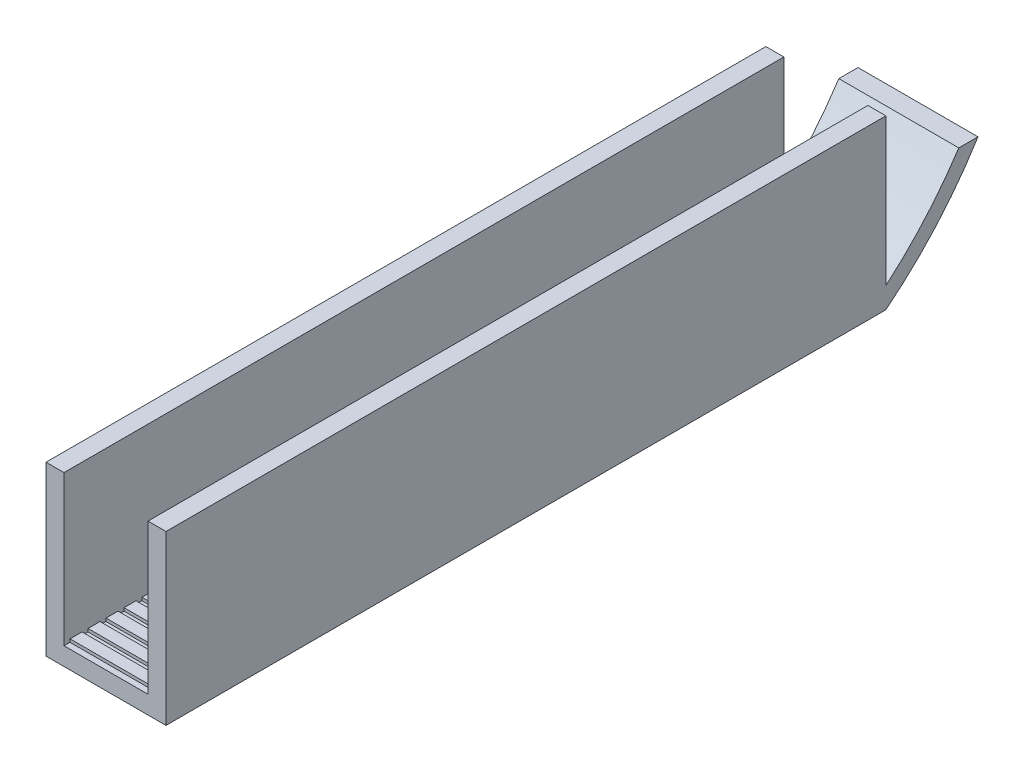
from build123d import *

# Parameters (mm, degrees)
SKETCH1_W           = 200
SKETCH1_H           = 30
BOSS_EXTRUDE1_DEPTH = 1200
SKETCH2_W           = 200
SKETCH2_H           = 20
BOSS_EXTRUDE2_DEPTH = 5
BOSS_EXTRUDE3_DEPTH = 200
SKETCH5_W           = 30
SKETCH5_H           = 1200
BOSS_EXTRUDE5_DEPTH = 250


with BuildPart() as part:
    # Sketch1 → Boss-Extrude1 (new body)
    with BuildSketch(Plane.XY):
        with Locations((-100, 15)):
            Rectangle(SKETCH1_W, SKETCH1_H)
    extrude(amount=BOSS_EXTRUDE1_DEPTH)

    # Sketch2 → Boss-Extrude2 (add)
    with BuildSketch(Plane(origin=(0, 30, 0), x_dir=(1, 0, 0), z_dir=(0, 1, 0))):
        with Locations((-100, -10)):
            Rectangle(SKETCH2_W, SKETCH2_H)
        with Locations((-100, -40)):
            Rectangle(SKETCH2_W, SKETCH2_H)
        with Locations((-100, -70)):
            Rectangle(SKETCH2_W, SKETCH2_H)
        with Locations((-100, -100)):
            Rectangle(SKETCH2_W, SKETCH2_H)
        with Locations((-100, -130)):
            Rectangle(SKETCH2_W, SKETCH2_H)
        with Locations((-100, -160)):
            Rectangle(SKETCH2_W, SKETCH2_H)
        with Locations((-100, -190)):
            Rectangle(SKETCH2_W, SKETCH2_H)
        with Locations((-100, -220)):
            Rectangle(SKETCH2_W, SKETCH2_H)
        with Locations((-100, -250)):
            Rectangle(SKETCH2_W, SKETCH2_H)
        with Locations((-100, -280)):
            Rectangle(SKETCH2_W, SKETCH2_H)
        with Locations((-100, -310)):
            Rectangle(SKETCH2_W, SKETCH2_H)
        with Locations((-100, -340)):
            Rectangle(SKETCH2_W, SKETCH2_H)
        with Locations((-100, -370)):
            Rectangle(SKETCH2_W, SKETCH2_H)
        with Locations((-100, -400)):
            Rectangle(SKETCH2_W, SKETCH2_H)
        with Locations((-100, -430)):
            Rectangle(SKETCH2_W, SKETCH2_H)
        with Locations((-100, -460)):
            Rectangle(SKETCH2_W, SKETCH2_H)
        with Locations((-100, -490)):
            Rectangle(SKETCH2_W, SKETCH2_H)
        with Locations((-100, -520)):
            Rectangle(SKETCH2_W, SKETCH2_H)
        with Locations((-100, -550)):
            Rectangle(SKETCH2_W, SKETCH2_H)
        with Locations((-100, -580)):
            Rectangle(SKETCH2_W, SKETCH2_H)
        with Locations((-100, -610)):
            Rectangle(SKETCH2_W, SKETCH2_H)
        with Locations((-100, -640)):
            Rectangle(SKETCH2_W, SKETCH2_H)
        with Locations((-100, -670)):
            Rectangle(SKETCH2_W, SKETCH2_H)
        with Locations((-100, -700)):
            Rectangle(SKETCH2_W, SKETCH2_H)
        with Locations((-100, -730)):
            Rectangle(SKETCH2_W, SKETCH2_H)
        with Locations((-100, -760)):
            Rectangle(SKETCH2_W, SKETCH2_H)
        with Locations((-100, -790)):
            Rectangle(SKETCH2_W, SKETCH2_H)
        with Locations((-100, -820)):
            Rectangle(SKETCH2_W, SKETCH2_H)
        with Locations((-100, -850)):
            Rectangle(SKETCH2_W, SKETCH2_H)
        with Locations((-100, -880)):
            Rectangle(SKETCH2_W, SKETCH2_H)
        with Locations((-100, -910)):
            Rectangle(SKETCH2_W, SKETCH2_H)
        with Locations((-100, -940)):
            Rectangle(SKETCH2_W, SKETCH2_H)
        with Locations((-100, -970)):
            Rectangle(SKETCH2_W, SKETCH2_H)
        with Locations((-100, -1000)):
            Rectangle(SKETCH2_W, SKETCH2_H)
        with Locations((-100, -1030)):
            Rectangle(SKETCH2_W, SKETCH2_H)
        with Locations((-100, -1060)):
            Rectangle(SKETCH2_W, SKETCH2_H)
        with Locations((-100, -1090)):
            Rectangle(SKETCH2_W, SKETCH2_H)
        with Locations((-100, -1120)):
            Rectangle(SKETCH2_W, SKETCH2_H)
        with Locations((-100, -1150)):
            Rectangle(SKETCH2_W, SKETCH2_H)
        with Locations((-100, -1180)):
            Rectangle(SKETCH2_W, SKETCH2_H)
    extrude(amount=BOSS_EXTRUDE2_DEPTH)

    # Sketch3 → Boss-Extrude3 (add)
    with BuildSketch(Plane(origin=(0, 0, 0), x_dir=(0, 0, -1), z_dir=(1, 0, 0))):
        with BuildLine():
            Line((121.535209025, 172.957157936), (153.547498251, 172.957157936))
            ThreePointArc((153.547498251, 172.957157936), (84.214276957, 79.873044696), (0, 0))
            Line((0, 0), (-44.824767416, 0))
            ThreePointArc((-44.824767416, 0), (46.406337039, 78.734560026), (121.535209025, 172.957157936))
        make_face()
    extrude(amount=-BOSS_EXTRUDE3_DEPTH)

    # Sketch5 → Boss-Extrude5 (add)
    with BuildSketch(Plane(origin=(0, 30, 0), x_dir=(1, 0, 0), z_dir=(0, 1, 0))):
        with Locations((-185, -600)):
            Rectangle(SKETCH5_W, SKETCH5_H)
        with Locations((-15, -600)):
            Rectangle(SKETCH5_W, SKETCH5_H)
    extrude(amount=BOSS_EXTRUDE5_DEPTH)


solid = part.part
